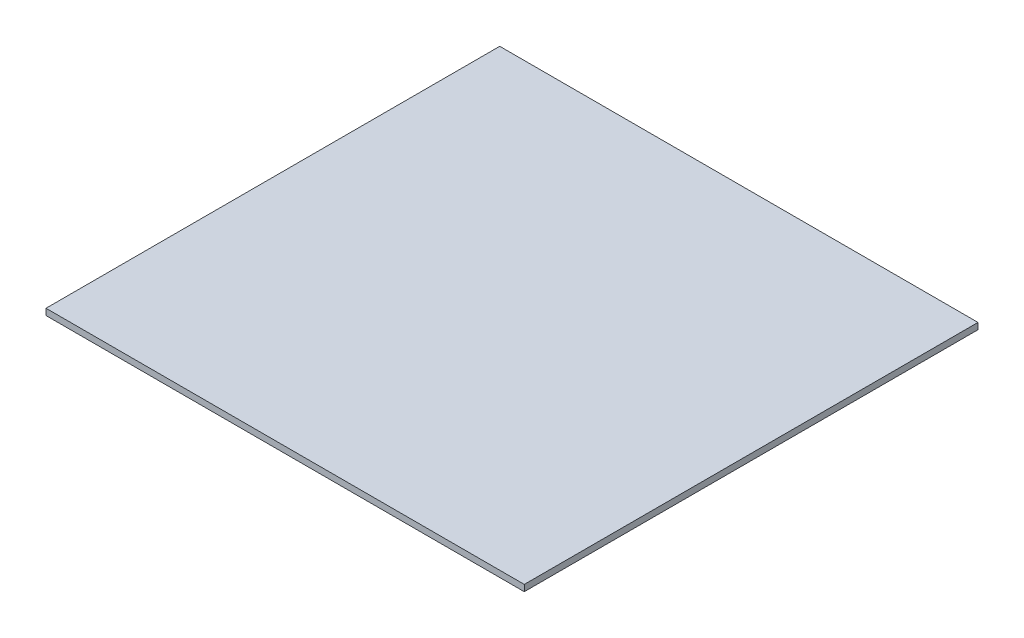
SolidWorks part; units mm, degrees
material "Q235A"
ref_plane "前视基准面" through (0, 0, 0) normal (0, 0, 1) x (1, 0, 0)
ref_plane "上视基准面" through (0, 0, 0) normal (0, 1, 0) x (1, 0, 0)
ref_plane "右视基准面" through (0, 0, 0) normal (1, 0, 0) x (0, 0, -1)
sketch3d "参数化"
  line L0 (-30.6165, 0, 0) -> (30.6165, 0, 0)
  line L1 (0, -14.0929, 0) -> (0, 14.0929, 0)
  line L2 (0, 0, 21.6949) -> (0, 0, -21.6949)
  point P4 (0, 0, 0)
  point P8 (0, 0, 0)
  point P11 (0, 0, 0)
sketch "草图1" plane through (0, 0, 0) normal (0, 1, 0) x (1, 0, 0)
  line L1 (-565, -536) -> (565, -536)
  line L2 (-565, -536) -> (-565, 536)
  line L3 (-565, 536) -> (565, 536)
  line L4 (565, -536) -> (565, 536)
  line L5 (-565, -536) -> (565, 536) construction
  line L6 (-565, 536) -> (565, -536) construction
  point P0 (0, 0)
extrude "凸台-拉伸1" add sketch "草图1" along normal blind 15
sketch "草图2" plane through (0, 15, 0) normal (0, 1, 0) x (1, 0, 0)
  line L0 (-565, -536) -> (565, -536) construction
  line L1 (-300, -536) -> (450, -536)
  line L2 (-300, -536) -> (-300, -586)
  line L3 (-300, -586) -> (450, -586)
  line L4 (450, -536) -> (450, -586)
  line L5 (0, 0) -> (0, -586) construction
extrude "凸台-拉伸2" [suppressed] add sketch "草图2" against normal blind 15
equation "\"A\" =1195"
equation "\"B\" =1155"
equation "\"CH\" = 2300"
equation "\"OP\" =750"
equation "\"OPH\" = 2100"
equation "\"QB\" = 50"
equation "\"DK\" = 40"
equation "\"WCOP\" =0"
equation "\"HCOP\" =4"
equation "\"FJ\" = 2"
equation "\"DH\" = 16"
equation "\"LG\" = 1"
equation "\"DD\" = 2"
equation "\"C\" =545"
equation "\"PX\" =-75"
equation "\"LZ\" = 350"
equation "\"LJ\" = 1158"
equation "\"LLK\" = 310"
equation "\"FS\" = 0"
equation "\"T\" = 80"
equation "\"D1@草图1\"=\"A\" - 60 - 5"
equation "\"D2@草图1\"=\"B\" - \"QB\" -30 -3"
equation "\"D1@草图2\"=\"OP\""
equation "\"D2@草图2\"=\"QB\""
equation "\"D3@草图2\"=\"OP\" / 2 + \"PX\""
equation "\"凸台-拉伸2\"= IIF ( \"LG\" = 1 , \"suppressed\" , \"unsuppressed\" )"
